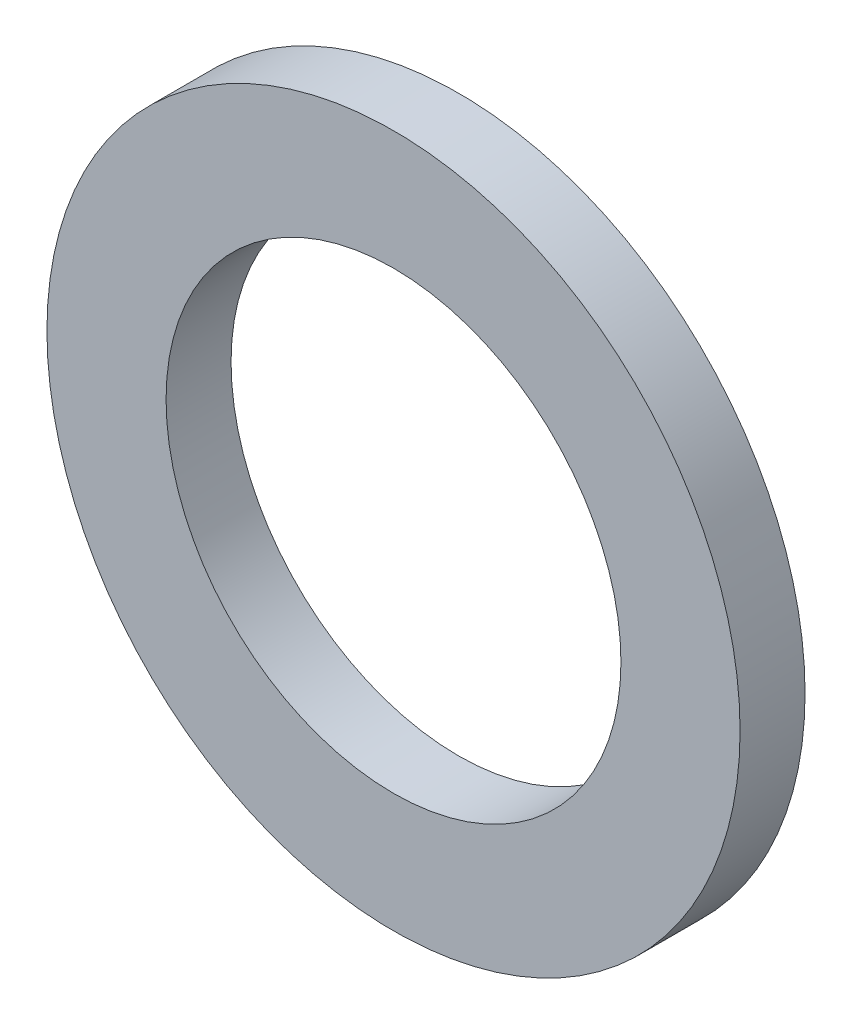
SolidWorks part; units mm, degrees
ref_plane "前视基准面" through (0, 0, 0) normal (0, 0, 1) x (1, 0, 0)
ref_plane "上视基准面" through (0, 0, 0) normal (0, 1, 0) x (1, 0, 0)
ref_plane "右视基准面" through (0, 0, 0) normal (1, 0, 0) x (0, 0, -1)
sketch "尺寸草图" plane through (0, 0, 0) normal (0, 0, 1) x (1, 0, 0)
  line L0 (0, 0) -> (1.5, 0) construction
  circle A0 centre (0, 0) radius 8
  circle A1 centre (0, 0) radius 5.25
  dimension "D" = 16
  dimension "(d)" = 10.5
  dimension "δ" = 1.5
extrude "拉伸1" add sketch "尺寸草图" along normal blind 1.5
